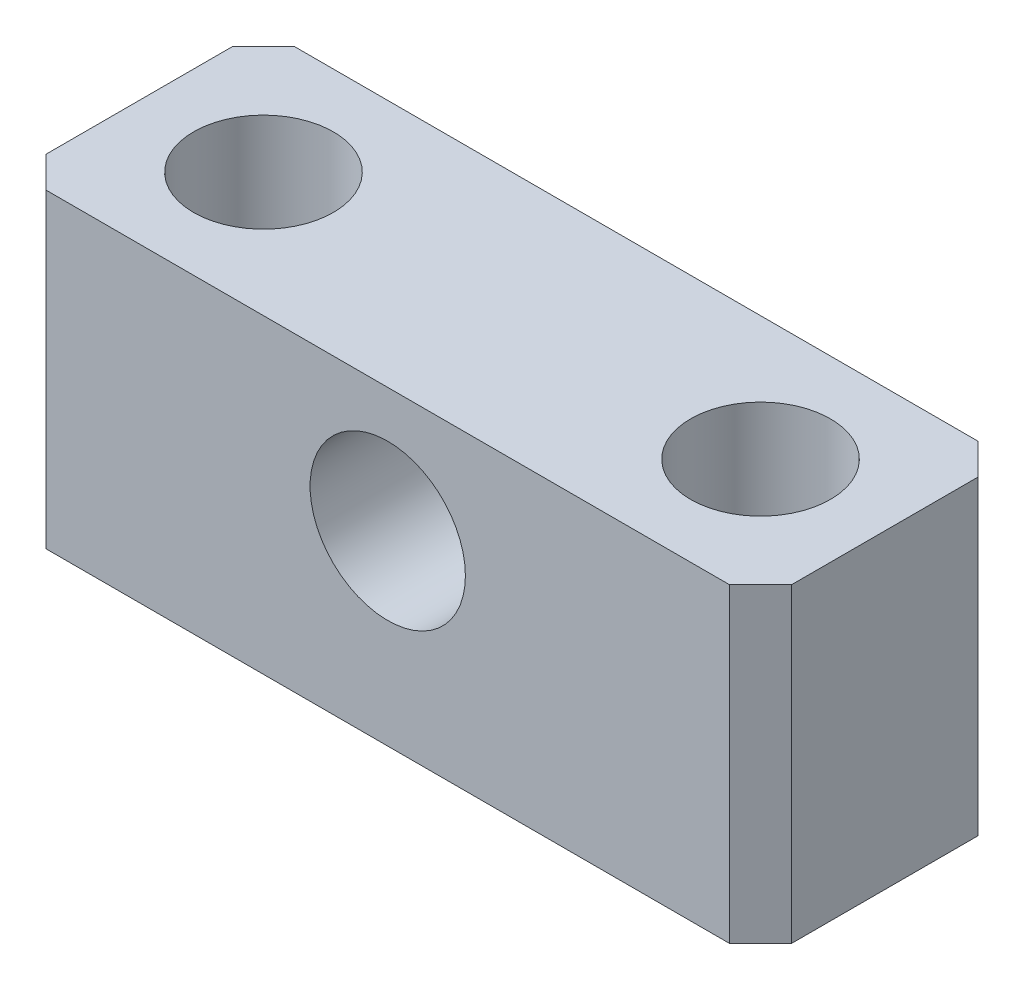
from build123d import *

# Parameters (mm, degrees)
SKETCH1_W                  = 24
SKETCH1_H                  = 10
BOSS_EXTRUDE1_DEPTH        = 4
F_4_5_4_5_DIAMETER_HOLE1_D = 4.5
CHAMFER1_SIZE              = 1
F_5_0_5_DIAMETER_HOLE1_D   = 5


with BuildPart() as part:
    # Sketch1 → Boss-Extrude1 (new, symmetric)
    with BuildSketch(Plane.XY):
        Rectangle(SKETCH1_W, SKETCH1_H)
    extrude(amount=BOSS_EXTRUDE1_DEPTH, both=True)

    # Ø4.5 (4.5) Diameter Hole1 (through all)
    with Locations(Plane(origin=(0, 5, 0), x_dir=(1, 0, 0), z_dir=(0, 1, 0))):
        with Locations((-8, 0), (8, 0)):
            Hole(F_4_5_4_5_DIAMETER_HOLE1_D / 2)

    # Chamfer1
    chamfer1_edges = [part.edges().sort_by_distance(p)[0] for p in [
        (-12, 0, 4),
        (12, 0, 4),
        (-12, 0, -4),
        (12, 0, -4),
    ]]
    chamfer(chamfer1_edges, length=CHAMFER1_SIZE)

    # Ø5.0 (5) Diameter Hole1 (through all)
    with Locations(Plane.XY.offset(4)):
        with Locations((0, 1)):
            Hole(F_5_0_5_DIAMETER_HOLE1_D / 2)


solid = part.part
